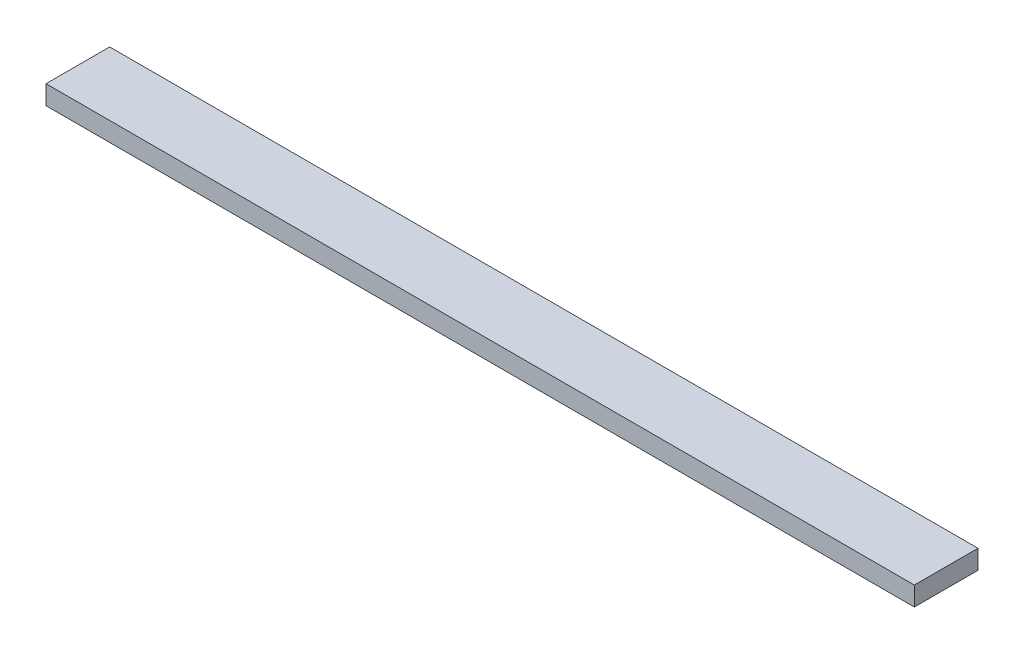
from build123d import *

# Parameters (mm, degrees)
SKETCH1_W           = 1364
SKETCH1_H           = 100
BOSS_EXTRUDE1_DEPTH = 30


with BuildPart() as part:
    # Sketch1 → Boss-Extrude1 (new body)
    with BuildSketch(Plane(origin=(0, 0, 0), x_dir=(1, 0, 0), z_dir=(0, 1, 0))):
        Rectangle(SKETCH1_W, SKETCH1_H)
    extrude(amount=BOSS_EXTRUDE1_DEPTH)


solid = part.part
